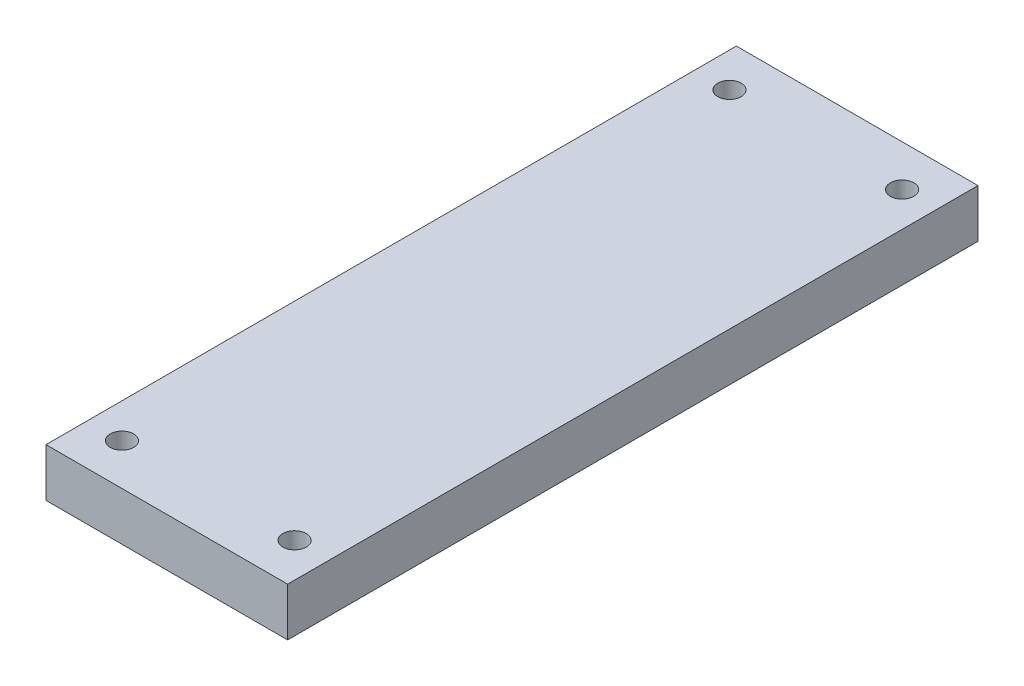
SolidWorks part; units mm, degrees
material "Q235"
ref_plane "Front Plane" through (0, 0, 0) normal (0, 0, 1) x (1, 0, 0)
ref_plane "Top Plane" through (0, 0, 0) normal (0, 1, 0) x (1, 0, 0)
ref_plane "Right Plane" through (0, 0, 0) normal (1, 0, 0) x (0, 0, -1)
sketch "Sketch1" plane through (0, 0, 0) normal (0, 1, 0) x (1, 0, 0)
  line L1 (0, 0) -> (70, 0)
  line L2 (0, 0) -> (0, 200)
  line L3 (0, 200) -> (70, 200)
  line L4 (70, 0) -> (70, 200)
  point P7 (70, 200)
  point P12 (70, 0)
  point P15 (0, 0)
  dimension "D1" = 70
  dimension "D2" = 200
extrude "Boss-Extrude1" add sketch "Sketch1" along normal blind 14
hole_wizard "Hole size (%based on) socket head cap screw type1" positions "Sketch2" profile "Sketch3" counterbore size "M8" standard "GB"
sketch "Sketch2" plane through (0, 14, 0) normal (0, 1, 0) x (1, 0, 0)
  line L0 (0, 100) -> (70, 100) construction
  line L1 (0, 200) -> (0, 0) construction
  line L2 (70, 0) -> (70, 200) construction
  line L5 (35, 200) -> (35, 168.287) construction
  line L6 (70, 200) -> (0, 200) construction
  point P0 (10, 155)
  point P2 (60, 155)
  point P4 (60, 45)
  point P6 (10, 45)
  dimension "D1" = 50
  dimension "D2" = 110
sketch "Sketch3" plane through (10, 14, -155) normal (1, 0, 0) x (0, 0, 1)
  line L0 (0, 0) -> (0, 14)
  line L1 (0, 14) -> (4.5, 14)
  line L3 (4.5, 14) -> (4.5, 9)
  line L4 (4.5, 9) -> (7.5, 9)
  line L5 (7.5, 9) -> (7.5, 0)
  line L7 (7.5, 0) -> (0, 0)
  line L11 (0, -6.35) -> (0, 107.95) construction
  dimension "通孔孔直径" = 9
  dimension "通孔孔深度" = 14
  dimension "柱形沉头孔直径" = 15
  dimension "柱形沉头孔深度" = 9
hole_wizard "M8 Tapped Hole1" positions "Sketch4" profile "Sketch5" tap size "M8" standard "GB" end condition through all
sketch "Sketch4" plane through (0, 0, 0) normal (0, -1, 0) x (-1, 0, 0)
  line L0 (-35, 200) -> (-35, 156.1442) construction
  line L1 (-70, 200) -> (0, 200) construction
  line L3 (0, 100) -> (-45.6733, 100) construction
  line L4 (0, 200) -> (0, 0) construction
  point P0 (-60, 188)
  point P2 (-10, 188)
  point P4 (-10, 12)
  point P6 (-60, 12)
  dimension "D1" = 50
  dimension "D2" = 12
sketch "Sketch5" plane through (60, 0, -188) normal (1, 0, 0) x (0, 0, -1)
  line L0 (0, 0) -> (0, 14)
  line L1 (0, 14) -> (3.4, 14)
  line L2 (3.4, 14) -> (3.4, 0)
  line L5 (3.4, 0) -> (0, 0)
  line L11 (0, -6.35) -> (0, 107.95) construction
  dimension "通孔螺纹孔钻头直径" = 6.8
  dimension "通孔螺纹孔钻头深度" = 14
cosmetic thread "Hole thread1" parameters "D2"=8
cosmetic thread "Hole thread2" parameters "D2"=8
cosmetic thread "Hole thread3" parameters "D2"=8
cosmetic thread "Hole thread4" parameters "D2"=8
